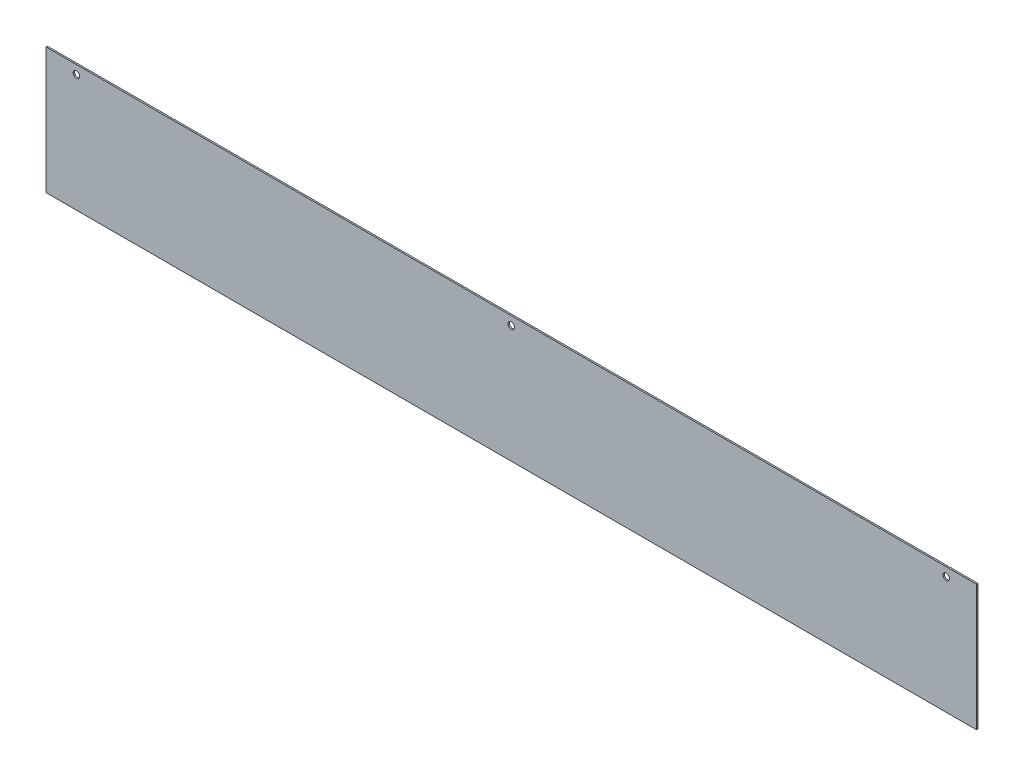
SolidWorks part; units mm, degrees
material "45#"
ref_plane "Front Plane" through (0, 0, 0) normal (0, 0, 1) x (1, 0, 0)
ref_plane "Top Plane" through (0, 0, 0) normal (0, 1, 0) x (1, 0, 0)
ref_plane "Right Plane" through (0, 0, 0) normal (1, 0, 0) x (0, 0, -1)
sketch "Sketch1" plane through (0, 0, 0) normal (0, 1, 0) x (1, 0, 0)
  line L0 (321, 0.5) -> (-321, -0.5) construction
  line L1 (-321, 0.5) -> (321, 0.5)
  line L2 (-321, 0.5) -> (-321, -0.5)
  line L3 (-321, -0.5) -> (321, -0.5)
  line L4 (321, 0.5) -> (321, -0.5)
  dimension "D1" = 642
  dimension "D2" = 1
extrude "Extrude1" add sketch "Sketch1" along normal mid plane 87
sketch "Sketch2" plane through (0, 0, 0.5) normal (0, 0, 1) x (1, 0, 0)
  line L0 (0, 43.5) -> (0, -43.5) construction
  line L1 (-321, 43.5) -> (321, 43.5) construction
  line L2 (-321, -43.5) -> (321, -43.5) construction
  line L3 (-300, 37.5) -> (0, 37.5) construction
  circle A0 centre (-300, 37.5) radius 2.25
  circle A2 centre (0, 37.5) radius 2.25
  circle A4 centre (300, 37.5) radius 2.25
  dimension "D1" = 4.5
  dimension "D2" = 6
  dimension "D3" = 600
extrude "Cut-Extrude1" cut sketch "Sketch2" against normal through all
